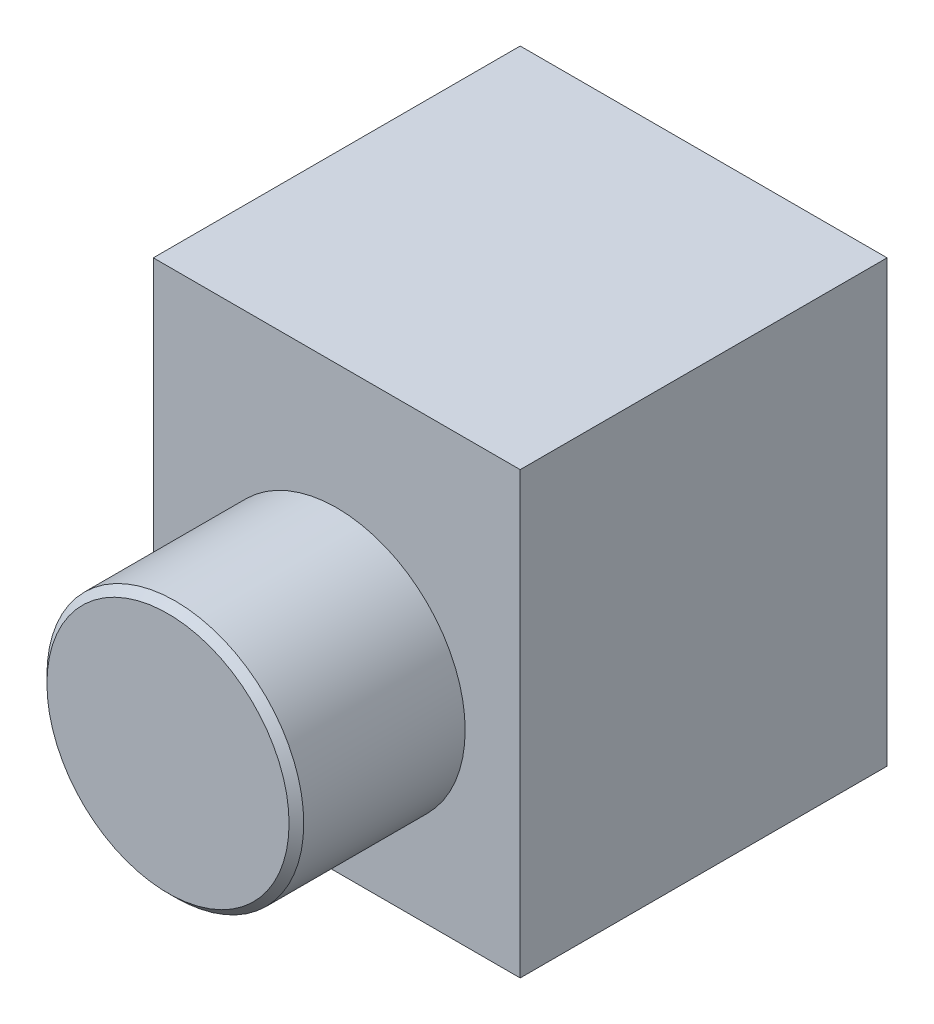
SolidWorks part; units mm, degrees
ref_plane "前视基准面" through (0, 0, 0) normal (0, 0, 1) x (1, 0, 0)
ref_plane "上视基准面" through (0, 0, 0) normal (0, 1, 0) x (1, 0, 0)
ref_plane "右视基准面" through (0, 0, 0) normal (1, 0, 0) x (0, 0, -1)
other "Configuration Table"
sketch "草图1" plane through (0, 0, 0) normal (0, 0, 1) x (1, 0, 0)
  line L1 (-25, -30) -> (25, -30)
  line L2 (-25, -30) -> (-25, 30)
  line L3 (-25, 30) -> (25, 30)
  line L4 (25, -30) -> (25, 30)
  line L5 (0, 30) -> (0, -30) construction
  line L6 (-25, 0) -> (25, 0) construction
  point P0 (0, 0)
  dimension "D1" = 50
  dimension "D2" = 60
extrude "凸台-拉伸1" add sketch "草图1" along normal blind 50
sketch "草图2" plane through (0, 0, 50) normal (0, 0, 1) x (1, 0, 0)
  line L1 (-25, -30) -> (25, -30) construction
  circle A0 centre (0, -4.5) radius 17.5
  dimension "D1" = 35
  dimension "D2" = 25.5
  dimension "D3" = 4.5
extrude "凸台-拉伸2" add sketch "草图2" along normal blind 23
sketch "草图5" plane through (0, -30, 0) normal (0, -1, 0) x (-1, 0, 0)
  line L0 (25, 0) -> (-25, 0) construction
  line L1 (25, -50) -> (25, 0) construction
  point P0 (0, -25)
  dimension "D1" = 25
  dimension "D2" = 25
hole_wizard "M30x2.0 螺纹孔1" positions "草图5" profile "草图4" tap size "M30x2.0" standard "GB"
sketch "草图4" plane through (0, -30, 25) normal (1, 0, 0) x (0, 0, -1)
  line L0 (0, 0) -> (0, 28.412)
  line L1 (0, 28.412) -> (14, 20)
  line L2 (14, 20) -> (14, 0)
  line L5 (14, 0) -> (0, 0)
  line L10 (0, 28.412) -> (-14, 20) construction
  line L11 (0, -6.35) -> (0, 107.95) construction
  dimension "螺纹孔钻头直径" = 28
  dimension "螺纹孔钻头深度" = 20
  dimension "导头角度" = 118
cosmetic thread "孔螺纹线1" parameters "D1"=60, "D2"=30
chamfer "倒角1" distance 1 angle 45 1 edges at (17.5, -4.5, 73)
